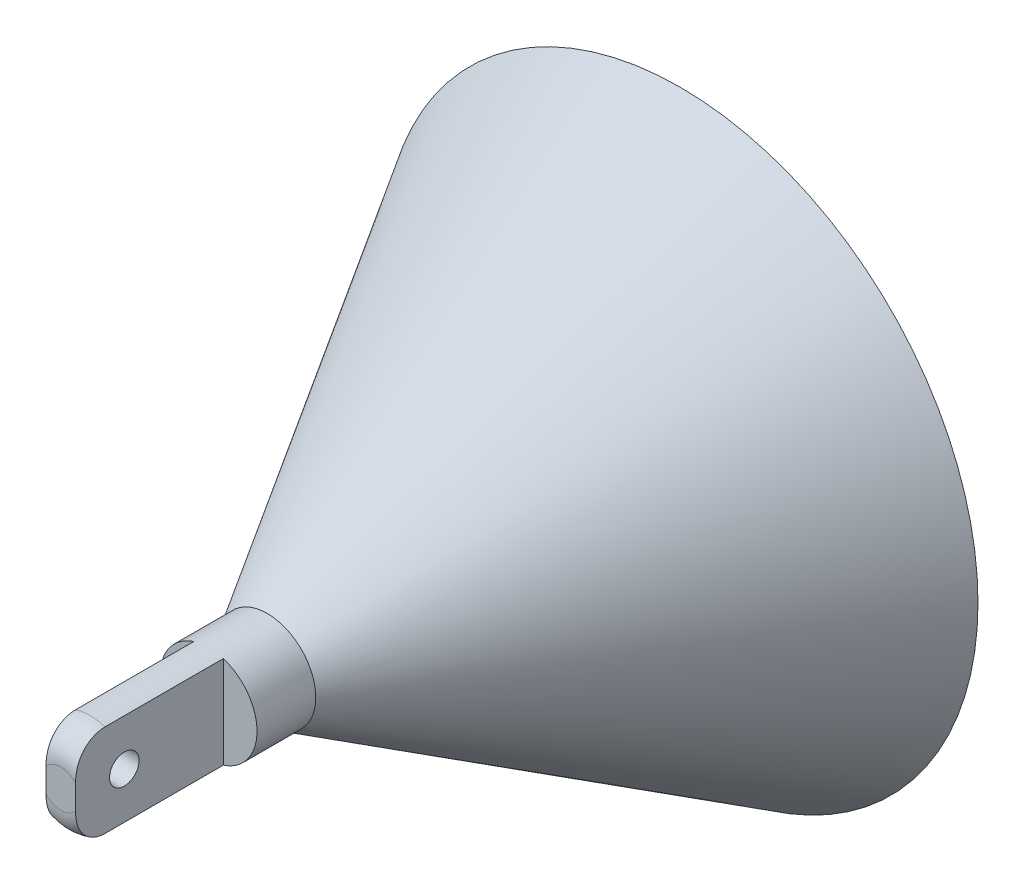
SolidWorks part; units mm, degrees
ref_plane "Front Plane" through (0, 0, 0) normal (0, 0, 1) x (1, 0, 0)
ref_plane "Top Plane" through (0, 0, 0) normal (0, 1, 0) x (1, 0, 0)
ref_plane "Right Plane" through (0, 0, 0) normal (1, 0, 0) x (0, 0, -1)
other "Configuration Table"
sketch "Sketch1" plane through (0, 0, 0) normal (0, 1, 0) x (1, 0, 0)
  line L0 (0, 0) -> (16.4028, 0)
  line L1 (16.4028, 0) -> (16.4028, 69.8741)
  line L2 (16.4028, 69.8741) -> (100.7142, 209.626)
  line L3 (100.7142, 209.626) -> (8.2014, 209.626)
  line L4 (0, 0) -> (0, 209.626)
  line L5 (0, 209.626) -> (8.2014, 209.626)
  dimension "D1" = 69.8741
revolve "Revolve1" add sketch "Sketch1" angle 360 about L4
sketch "Sketch2" plane through (0, 0, 0) normal (0, 0, 1) x (1, 0, 0)
  line L0 (0, -110.7856) -> (0, 110.7856) construction
  line L1 (-27.9585, 19.0057) -> (-5, 19.0057)
  line L2 (-27.9585, 19.0057) -> (-27.9585, -23.5718)
  line L3 (-27.9585, -23.5718) -> (-5, -23.5718)
  line L4 (-5, 19.0057) -> (-5, -23.5718)
  line L5 (5, 19.0057) -> (5, -23.5718)
  line L6 (27.9585, -23.5718) -> (5, -23.5718)
  line L7 (27.9585, 19.0057) -> (27.9585, -23.5718)
  line L8 (27.9585, 19.0057) -> (5, 19.0057)
  dimension "D1" = 5
extrude "Cut-Extrude1" cut sketch "Sketch2" against normal blind 50
sketch "Sketch3" plane through (5, 0, 0) normal (1, 0, 0) x (0, 0, -1)
  circle A0 centre (16.4984, 0) radius 5
  dimension "D1" = 10
extrude "Cut-Extrude2" cut sketch "Sketch3" against normal blind 50
fillet "Fillet1" radius 10 2 edges at (0, -16.4028, 0) (0, 16.4028, 0)
sketch "Sketch4" plane through (0, 0, 0) normal (1, 0, 0) x (0, 0, -1)
  line L0 (77.001, 14.0667) -> (233.1653, 99.1816)
  line L1 (233.1653, 99.1816) -> (233.1653, 0)
  line L2 (233.1653, 0) -> (77.001, 0)
  line L3 (77.001, 0) -> (77.001, 14.0667)
revolve "Cut-Revolve1" cut sketch "Sketch4" angle 360 about L2
